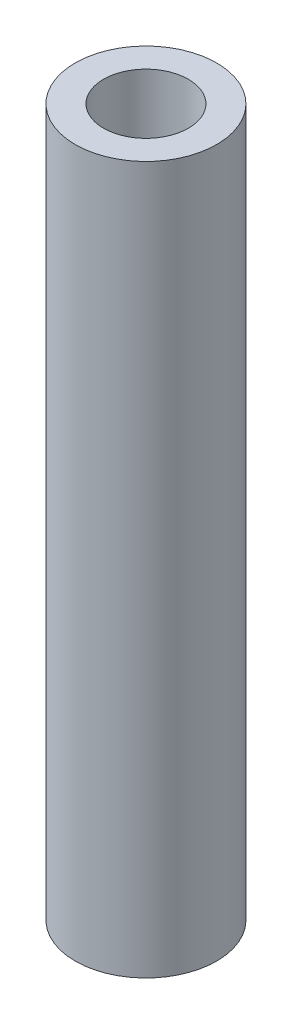
SolidWorks part; units mm, degrees
material "6061-T6 (SS)"
ref_plane "Front Plane" through (0, 0, 0) normal (0, 0, 1) x (1, 0, 0)
ref_plane "Top Plane" through (0, 0, 0) normal (0, 1, 0) x (1, 0, 0)
ref_plane "Right Plane" through (0, 0, 0) normal (1, 0, 0) x (0, 0, -1)
sketch "Sketch1" plane through (0, 0, 0) normal (0, 1, 0) x (1, 0, 0)
  circle A0 centre (0, 0) radius 2.5
  circle A1 centre (0, 0) radius 1.5
  dimension "D1" = 5
  dimension "D2" = 3
extrude "Boss-Extrude1" add sketch "Sketch1" along normal blind 25
cosmetic thread "Cosmetic Thread1" parameters "D1"=5, "D2"=4
sketch "Sketch2" plane through (0, 0, 0) normal (0, -1, 0) x (1, 0, 0)
  circle A0 centre (0, 0) radius 1.5 construction
  circle A1 centre (0, 0) radius 1.5
  circle A2 centre (0, 0) radius 0.5
  dimension "D1" = 1
extrude "Boss-Extrude2" add sketch "Sketch2" against normal blind 2
